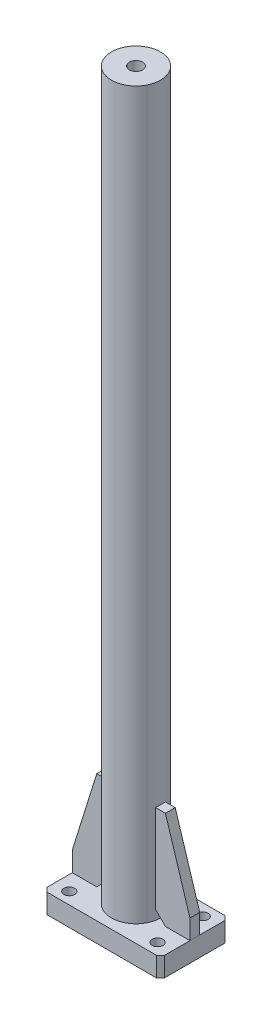
from build123d import *

# Parameters (mm, degrees)
SKETCH_1_R                  = 12.5
EXTRUDE_1_DEPTH             = 370
SKETCH_2_W                  = 60
SKETCH_2_H                  = 35
EXTRUDE_2_DEPTH             = 10
EXTRUDE_3_DEPTH             = 2.5
EXTRUDE_3_2_DEPTH           = 2.5
SKETCH_5_W                  = 2.75
SKETCH_5_H                  = 10.001
HOLE_WIZARD_M5_1_AT_2_COUNT = 2
HOLE_WIZARD_M5_1_AT_2_PITCH = 45
HOLE_WIZARD_M5_1_AT_3_COUNT = 2
HOLE_WIZARD_M5_1_AT_3_PITCH = 50.537115074
HOLE_WIZARD_M5_1_AT_4_COUNT = 2
HOLE_WIZARD_M5_1_AT_4_PITCH = 23
CHAMFER_1_SIZE              = 2


with BuildPart() as part:
    # 草图1 → 凸台-拉伸1 (new body)
    with BuildSketch(Plane(origin=(0, 0, 0), x_dir=(1, 0, 0), z_dir=(0, 1, 0))):
        with Locations(Location((0, 0, 0), (0, 0, 270))):
            Circle(SKETCH_1_R)
    extrude(amount=EXTRUDE_1_DEPTH)

    # 草图7 → M8 螺纹孔1 (revolve, cut)
    with BuildSketch(Plane(origin=(0, 370, 0), x_dir=(0, 0, 1), z_dir=(1, 0, 0))):
        Polygon((0, 0), (0, 21.792926105), (3.4, 19.75), (3.4, 0), align=None)
    revolve(axis=Axis((0, 376.35, 0), (0, -1, 0)), mode=Mode.SUBTRACT)


with BuildPart() as body_2:
    # 草图2 → 凸台-拉伸2 (new body)
    with BuildSketch(Plane.XZ):
        Rectangle(SKETCH_2_W, SKETCH_2_H)
    extrude(amount=EXTRUDE_2_DEPTH)

    # 草图5 → M5 间隙孔1 (revolve, cut)
    with BuildSketch(Plane(origin=(-22.5, -10, 11.5), x_dir=(0, 0, -1), z_dir=(1, 0, 0))):
        with Locations((1.375, 5.0005)):
            Rectangle(SKETCH_5_W, SKETCH_5_H)
    hole_wizard_m5_1 = revolve(axis=Axis((-22.5, -16.35, 11.5), (0, 1, 0)), mode=Mode.SUBTRACT)

    # M5 间隙孔1 at 2: M5 间隙孔1 ×2
    with Locations(*[(i * HOLE_WIZARD_M5_1_AT_2_PITCH, 0, 0) for i in range(1, HOLE_WIZARD_M5_1_AT_2_COUNT)]):
        add(hole_wizard_m5_1, mode=Mode.SUBTRACT)

    # M5 间隙孔1 at 3: M5 间隙孔1 ×2
    with Locations(*[Vector(0.8904346821960805, 0, -0.45511105978910815) * (i * HOLE_WIZARD_M5_1_AT_3_PITCH) for i in range(1, HOLE_WIZARD_M5_1_AT_3_COUNT)]):
        add(hole_wizard_m5_1, mode=Mode.SUBTRACT)

    # M5 间隙孔1 at 4: M5 间隙孔1 ×2
    with Locations(*[(0, 0, -i * HOLE_WIZARD_M5_1_AT_4_PITCH) for i in range(1, HOLE_WIZARD_M5_1_AT_4_COUNT)]):
        add(hole_wizard_m5_1, mode=Mode.SUBTRACT)

    # 倒角1
    chamfer_1_edges = [body_2.edges().sort_by_distance(p)[0] for p in [
        (-30, -5, 17.5),
        (30, -5, 17.5),
        (30, -5, -17.5),
        (-30, -5, -17.5),
    ]]
    chamfer(chamfer_1_edges, length=CHAMFER_1_SIZE)


with BuildPart() as body_3:
    # 草图3 → 凸台-拉伸3 (new, symmetric)
    with BuildSketch(Plane.XY):
        Polygon((30, 0), (30, 10), (17.5, 50), (12.5, 50), (12.5, 5), (17.5, 0), align=None)
    extrude(amount=EXTRUDE_3_DEPTH, both=True)


with BuildPart() as body_4:
    # 草图3 → Extrude 3 2 (new, symmetric)
    with BuildSketch(Plane.XY):
        Polygon((-12.5, 5), (-17.5, 0), (-30, 0), (-30, 10), (-17.5, 50), (-12.5, 50), align=None)
    extrude(amount=EXTRUDE_3_2_DEPTH, both=True)


solid = Compound([part.part, body_2.part, body_3.part, body_4.part])
